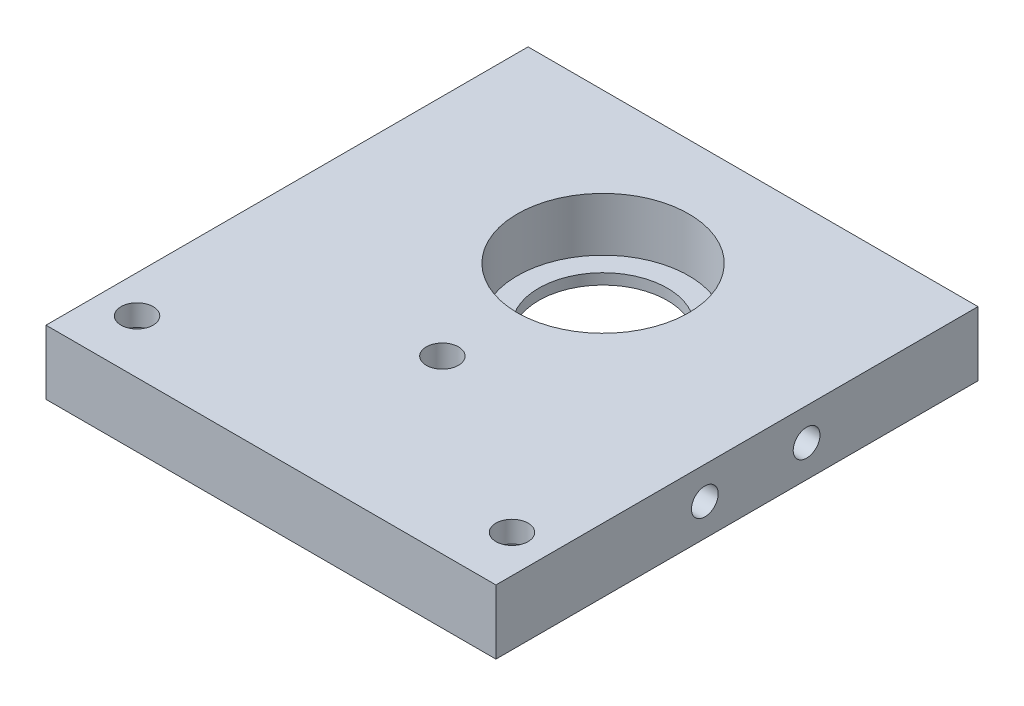
SolidWorks part; units mm, degrees
material "Q235B"
ref_plane "Front Plane" through (0, 0, 0) normal (0, 0, 1) x (1, 0, 0)
ref_plane "Top Plane" through (0, 0, 0) normal (0, 1, 0) x (1, 0, 0)
ref_plane "Right Plane" through (0, 0, 0) normal (1, 0, 0) x (0, 0, -1)
sketch "Sketch1" plane through (0, 0, 0) normal (0, 1, 0) x (1, 0, 0)
  line L1 (-21, 22.5) -> (21, 22.5)
  line L2 (-21, 22.5) -> (-21, -22.5)
  line L3 (-21, -22.5) -> (21, -22.5)
  line L4 (21, 22.5) -> (21, -22.5)
  line L5 (-21, 22.5) -> (21, -22.5) construction
  line L6 (-21, -22.5) -> (21, 22.5) construction
  circle A0 centre (0, 8.5) radius 6
  circle A1 centre (0, -6.5) radius 1.5
  point P0 (0, 0)
  dimension "D3" = 12
  dimension "D4" = 14
  dimension "D5" = 3
  dimension "D6" = 15
  dimension "D1" = 42
  dimension "D2" = 45
extrude "Boss-Extrude1" add sketch "Sketch1" along normal blind 6
sketch "Sketch3" plane through (0, 6, 0) normal (0, 1, 0) x (1, 0, 0)
  circle A0 centre (0, 8.5) radius 8
  dimension "D1" = 16
extrude "Cut-Extrude1" cut sketch "Sketch3" against normal blind 5
sketch "Sketch4" plane through (0, 6, 0) normal (0, 1, 0) x (1, 0, 0)
  line L0 (21, -22.5) -> (21, 22.5) construction
  line L1 (-21, 22.5) -> (-21, -22.5) construction
  line L2 (21, 22.5) -> (-21, 22.5) construction
  circle A0 centre (-17.5, -17.5) radius 1.5
  circle A1 centre (17.5, -17.5) radius 1.5
  dimension "D1" = 3
  dimension "D2" = 3.5
  dimension "D3" = 3.5
  dimension "D4" = 40
extrude "Cut-Extrude2" cut sketch "Sketch4" against normal through all
sketch "Sketch5" plane through (0, 0, 0) normal (0, -1, 0) x (1, 0, 0)
  circle A0 centre (17.5, 17.5) radius 2.5
  circle A1 centre (-17.5, 17.5) radius 2.5
  circle A2 centre (17.5, 17.5) radius 1.5 construction
  circle A3 centre (-17.5, 17.5) radius 1.5 construction
  dimension "D1" = 5
extrude "Cut-Extrude3" cut sketch "Sketch5" against normal blind 4
sketch "Sketch6" plane through (21, 0, 0) normal (1, 0, 0) x (0, 0, -1)
  line L0 (-22.5, 0) -> (22.5, 0) construction
  circle A0 centre (6.5, 3) radius 1
  circle A1 centre (-3, 3) radius 1
  dimension "D1" = 2
  dimension "D2" = 3
  dimension "D3" = 9.5
  dimension "D4" = 3
extrude "Cut-Extrude4" cut sketch "Sketch6" against normal blind 2
hole_wizard "M3 Tapped Hole1" positions "Sketch7" profile "Sketch8" tap size "M3" standard "GB"
sketch "Sketch7" plane through (21, 0, 0) normal (1, 0, 0) x (0, 0, -1)
  point P0 (6.5, 3)
  point P3 (-3, 3)
sketch "Sketch8" plane through (21, 3, -6.5) normal (0, 1, 0) x (0, 0, -1)
  line L0 (0, 0) -> (0, 8.2511)
  line L1 (0, 8.2511) -> (1.25, 7.5)
  line L2 (1.25, 7.5) -> (1.25, 0)
  line L5 (1.25, 0) -> (0, 0)
  line L10 (0, 8.2511) -> (-1.25, 7.5) construction
  line L11 (0, -6.35) -> (0, 107.95) construction
  dimension "螺纹孔钻头直径" = 2.5
  dimension "螺纹孔钻头深度" = 7.5
  dimension "导头角度" = 118
cosmetic thread "HoleThreadLine1" parameters "D1"=6, "D2"=3
cosmetic thread "HoleThreadLine2" parameters "D1"=6, "D2"=3
